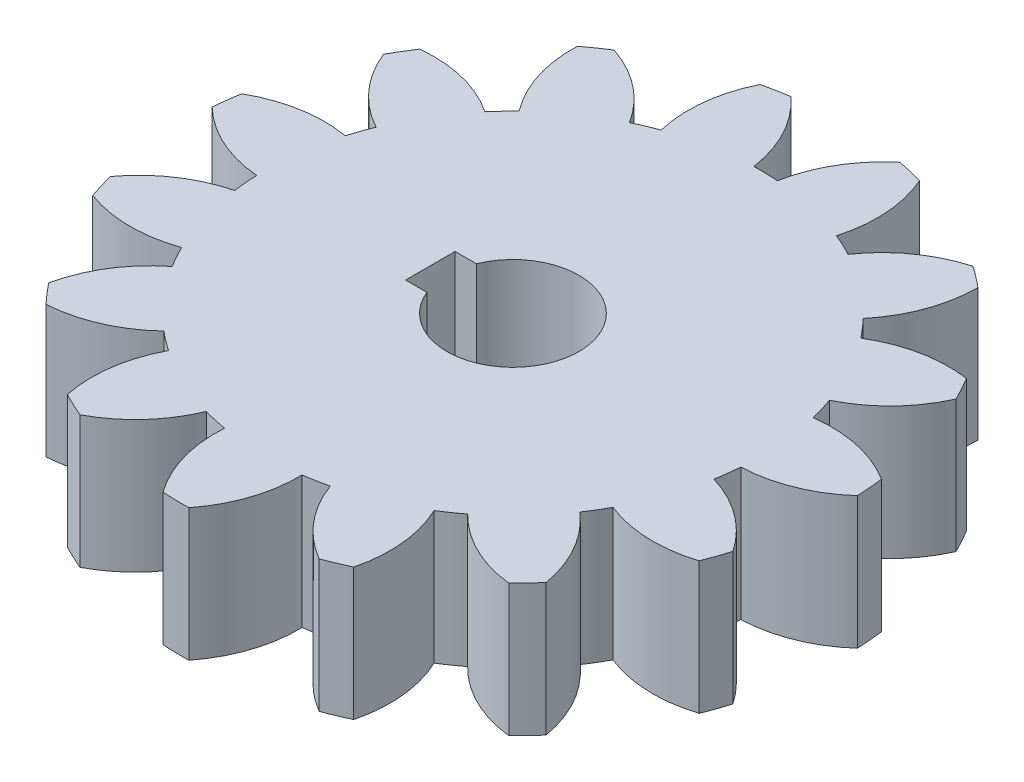
from build123d import *

# Parameters (mm, degrees)
BOSS_EXTRUDE1_DEPTH = 40


with BuildPart() as part:
    # Sketch1 → Boss-Extrude1 (new body)
    with BuildSketch(Plane(origin=(0, 0, 0), x_dir=(1, 0, 0), z_dir=(0, 1, 0))):
        with BuildLine():
            ThreePointArc((-47.041872024, 148.439333774), (-43.127492719, 149.266400751), (-39.183163492, 149.936230637))
            ThreePointArc((-39.183163492, 149.936230637), (-30.743985568, 139.078421622), (-26.480835029, 126.00412286))
            ThreePointArc((-26.480835029, 126.00412286), (-22.825050962, 126.015662102), (-19.173047629, 125.849042918))
            ThreePointArc((-19.173047629, 125.849042918), (-14.359080523, 138.730714445), (-5.466876345, 149.220730913))
            ThreePointArc((-5.466876345, 149.220730913), (-1.554514466, 148.384172695), (2.321253942, 147.391789516))
            ThreePointArc((2.321253942, 147.391789516), (5.614557811, 134.040164511), (4.191343232, 120.362218726))
            ThreePointArc((4.191343232, 120.362218726), (7.535761593, 118.885819009), (10.804262521, 117.248201234))
            ThreePointArc((10.804262521, 117.248201234), (20.441488139, 127.058176924), (32.831594958, 133.024498542))
            ThreePointArc((32.831594958, 133.024498542), (36.0654565, 130.668963645), (39.202508521, 128.185959468))
            ThreePointArc((39.202508521, 128.185959468), (36.780496177, 114.649135732), (29.91700321, 102.732584011))
            ThreePointArc((29.91700321, 102.732584011), (32.371775547, 100.023528258), (34.691620567, 97.198070883))
            ThreePointArc((34.691620567, 97.198070883), (47.485740835, 102.240116818), (61.231388266, 102.651112376))
            ThreePointArc((61.231388266, 102.651112376), (63.227585431, 99.183894183), (65.083496272, 95.639602987))
            ThreePointArc((65.083496272, 95.639602987), (57.364955653, 84.258220323), (46.247944585, 76.163542716))
            ThreePointArc((46.247944585, 76.163542716), (47.388618461, 72.690251279), (48.358685293, 69.165501552))
            ThreePointArc((48.358685293, 69.165501552), (62.097480586, 68.567802184), (74.821921313, 63.352406817))
            ThreePointArc((74.821921313, 63.352406817), (75.235293477, 59.373018851), (75.489159292, 55.380280784))
            ThreePointArc((75.489159292, 55.380280784), (63.808696192, 48.12228365), (50.360399232, 45.249123454))
            ThreePointArc((50.360399232, 45.249123454), (49.98974177, 41.612159976), (49.442297047, 37.997579146))
            ThreePointArc((49.442297047, 37.997579146), (61.750204846, 31.863482126), (71.253267468, 21.923485072))
            ThreePointArc((71.253267468, 21.923485072), (70.012338829, 18.119999666), (68.620263913, 14.369195412))
            ThreePointArc((68.620263913, 14.369195412), (54.997536515, 12.48955745), (41.543286381, 15.334710164))
            ThreePointArc((41.543286381, 15.334710164), (39.725387624, 12.162938671), (37.755089511, 9.083520601))
            ThreePointArc((37.755089511, 9.083520601), (46.503960743, -1.526332969), (51.142479402, -14.472215917))
            ThreePointArc((51.142479402, -14.472215917), (48.461817794, -17.442141584), (45.664504547, -20.302463895))
            ThreePointArc((45.664504547, -20.302463895), (32.455006176, -16.478736206), (21.321164945, -8.407223332))
            ThreePointArc((21.321164945, -8.407223332), (18.370356103, -10.565374735), (15.317887044, -12.577170684))
            ThreePointArc((15.317887044, -12.577170684), (18.994962393, -25.828240736), (17.966895072, -39.541548806))
            ThreePointArc((17.966895072, -39.541548806), (14.31001124, -41.164387605), (10.591140535, -42.639652259))
            ThreePointArc((10.591140535, -42.639652259), (0.078913465, -33.773716174), (-6.809376568, -21.871481045))
            ThreePointArc((-6.809376568, -21.871481045), (-10.382873838, -22.642848373), (-13.989714213, -23.239164406))
            ThreePointArc((-13.989714213, -23.239164406), (-16.02023448, -36.840220544), (-22.537125601, -48.94979819))
            ThreePointArc((-22.537125601, -48.94979819), (-26.53792322, -48.944946549), (-30.535324854, -48.780066887))
            ThreePointArc((-30.535324854, -48.780066887), (-36.532621062, -36.404923299), (-37.984311971, -22.729970496))
            ThreePointArc((-37.984311971, -22.729970496), (-41.562607528, -21.981177331), (-45.10016375, -21.058904988))
            ThreePointArc((-45.10016375, -21.058904988), (-52.487184233, -32.658201045), (-63.366069475, -41.07019228))
            ThreePointArc((-63.366069475, -41.07019228), (-67.019006626, -39.438489092), (-70.603752131, -37.661974304))
            ThreePointArc((-70.603752131, -37.661974304), (-71.049130479, -23.917397964), (-66.813211718, -10.834251061))
            ThreePointArc((-66.813211718, -10.834251061), (-69.777585752, -8.694770544), (-72.634182213, -6.413379092))
            ThreePointArc((-72.634182213, -6.413379092), (-84.100419961, -14.005291403), (-97.460241234, -17.265186521))
            ThreePointArc((-97.460241234, -17.265186521), (-100.133691899, -14.288768092), (-102.68594621, -11.207793723))
            ThreePointArc((-102.68594621, -11.207793723), (-97.502396736, 1.529653253), (-88.311297141, 11.758799301))
            ThreePointArc((-88.311297141, 11.758799301), (-90.149182451, 14.919031553), (-91.830887671, 18.165068806))
            ThreePointArc((-91.830887671, 18.165068806), (-105.39372601, 15.89325085), (-118.924448847, 18.349117329))
            ThreePointArc((-118.924448847, 18.349117329), (-120.156149117, 22.155601214), (-121.234604278, 26.008306704))
            ThreePointArc((-121.234604278, 26.008306704), (-111.318409777, 35.53620402), (-98.761353966, 41.142636931))
            ThreePointArc((-98.761353966, 41.142636931), (-99.154963485, 44.777188051), (-99.370995354, 48.426601775))
            ThreePointArc((-99.370995354, 48.426601775), (-112.685296321, 51.867696137), (-124.047335819, 59.614682589))
            ThreePointArc((-124.047335819, 59.614682589), (-123.624313529, 63.593056285), (-123.042494845, 67.551325117))
            ThreePointArc((-123.042494845, 67.551325117), (-110.108255432, 72.222212767), (-96.356472432, 72.236529359))
            ThreePointArc((-96.356472432, 72.236529359), (-95.237747499, 75.71695244), (-93.950752144, 79.138725848))
            ThreePointArc((-93.950752144, 79.138725848), (-104.714352145, 87.697736052), (-111.943108455, 99.396318139))
            ThreePointArc((-111.943108455, 99.396318139), (-109.938508001, 102.858684692), (-107.797017208, 106.238096225))
            ThreePointArc((-107.797017208, 106.238096225), (-94.081180381, 105.244335301), (-81.512478404, 99.664060105))
            ThreePointArc((-81.512478404, 99.664060105), (-79.074856723, 102.388558378), (-76.507367333, 104.991035762))
            ThreePointArc((-76.507367333, 104.991035762), (-82.859142143, 117.188031187), (-84.704697628, 130.815417788))
            ThreePointArc((-84.704697628, 130.815417788), (-81.46513264, 133.163102566), (-78.134252951, 135.379325845))
            ThreePointArc((-78.134252951, 135.379325845), (-66.008411502, 128.892746639), (-56.796033303, 118.682759932))
            ThreePointArc((-56.796033303, 118.682759932), (-53.461001807, 120.180242893), (-50.056960623, 121.513432271))
            ThreePointArc((-50.056960623, 121.513432271), (-50.898630674, 135.239441602), (-47.041872024, 148.439333774))
        make_face()
        with BuildLine():
            Line((-42.956778148, 58.532544108), (-49.41628193, 58.532544108))
            Line((-49.41628193, 58.532544108), (-49.41628193, 43.532544108))
            Line((-49.41628193, 43.532544108), (-42.956778148, 43.532544108))
            ThreePointArc((-42.956778148, 43.532544108), (-4.41628193, 51.032544108), (-42.956778148, 58.532544108))
        make_face(mode=Mode.SUBTRACT)
    extrude(amount=BOSS_EXTRUDE1_DEPTH)


solid = part.part
